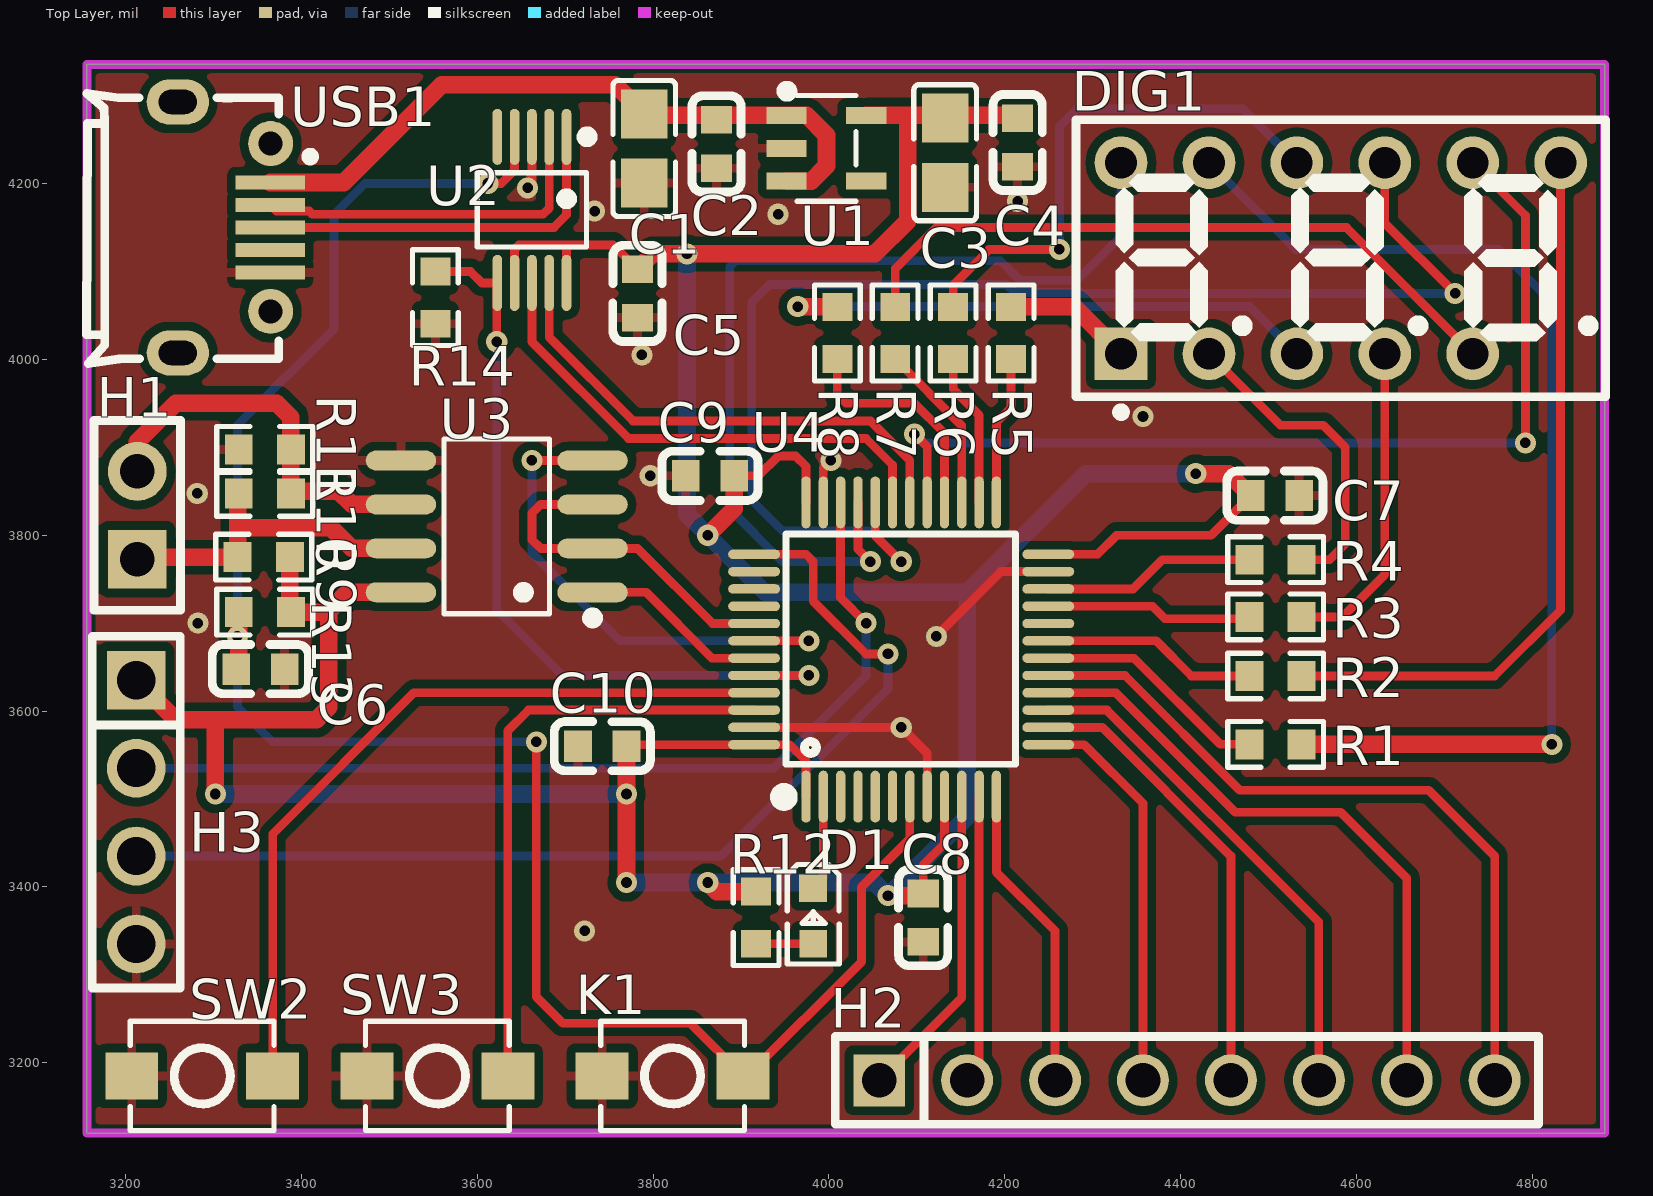
[diagram p0: Top Layer view]
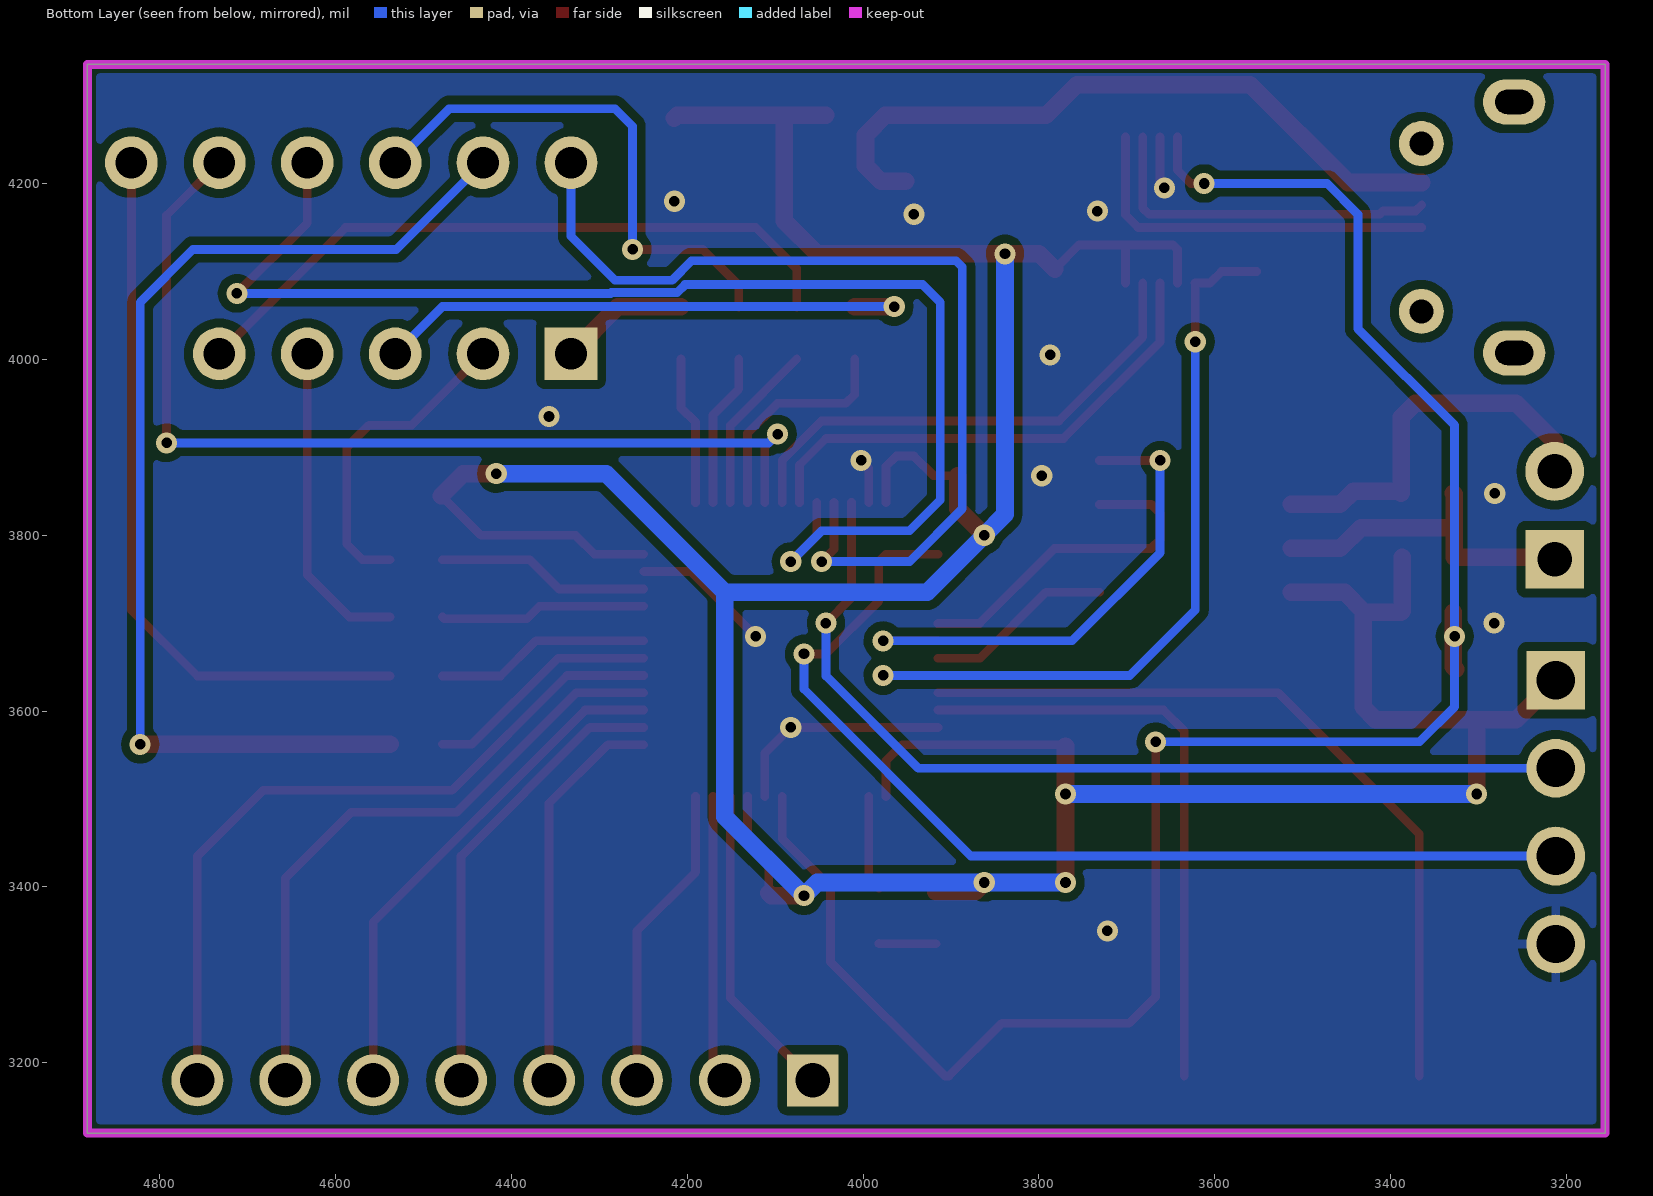
[diagram p1: Bottom Layer view, seen from below]
# Altium PCB MISC49919.pcbdoc
Units mil, origin at the board's own origin, x right, y up, seen from the top; angles counter-clockwise.
Board outline 1726.16 x 1215.5 mil, 2 copper layers (Top Layer, Bottom Layer), stack 62.206 mil thick; 37 components, 48 nets, 161 pads, 38 vias.

## Layer stack, top to bottom
Top Solder Mask Layer: solder mask 0.394, Dk 3.3
Top Layer: signal copper 1.379
Dielectric1: surface 59.449, FR4, Dk 4.5
Bottom Layer: signal copper 1.378
Bottom Solder Mask Layer: solder mask 0.394, Dk 3.3

## Board outline
3156.11,4335.5 3156.11,3120 4882.28,3120 4882.28,4335.5

## Design rules (kind name [scope] priority, off if disabled: settings)
BoardOutlineClearance copperThickness2oz_1 [All] p2 off: genericclearance=7.99 ignorepadtopadclearanceinfootprint=FALSE except(0: Arc-SplitContinuation Track-SplitContinuation SMDPad-SplitContinuation THPad-SplitContinuation Via-SplitContinuation Fill-SplitContinuation Region-SplitContinuation Poly-SplitContinuation Text-SplitContinuation Hole-SplitContinuation; 5.98: Arc-CutoutEdge SMDPad-CutoutEdge THPad-CutoutEdge Via-CutoutEdge Fill-CutoutEdge Region-CutoutEdge Text-CutoutEdge; 6.93: Hole-OutlineEdge Hole-CutoutEdge; 10: Poly-OutlineEdge Poly-CutoutEdge; 11.81: Arc-OutlineEdge Track-OutlineEdge SMDPad-OutlineEdge THPad-OutlineEdge Via-OutlineEdge Fill-OutlineEdge Region-OutlineEdge Text-OutlineEdge Track-CutoutEdge)
BoardOutlineClearance copperThickness1oz_1 [All] p4: genericclearance=4.02 ignorepadtopadclearanceinfootprint=FALSE except(0: Arc-SplitContinuation Track-SplitContinuation SMDPad-SplitContinuation THPad-SplitContinuation Via-SplitContinuation Fill-SplitContinuation Region-SplitContinuation Poly-SplitContinuation Text-SplitContinuation Hole-SplitContinuation; 6: SMDPad-CutoutEdge THPad-CutoutEdge Via-CutoutEdge Fill-CutoutEdge Region-CutoutEdge Text-CutoutEdge; 6.93: Hole-OutlineEdge Hole-CutoutEdge; 10: Poly-OutlineEdge Poly-CutoutEdge; 11.8: Arc-OutlineEdge Track-OutlineEdge SMDPad-OutlineEdge THPad-OutlineEdge Via-OutlineEdge Fill-OutlineEdge Region-OutlineEdge Text-OutlineEdge; 11.81: Arc-CutoutEdge Track-CutoutEdge)
Clearance copperThickness2oz [All] p1 off: gap=7.99 ignorepadtopadclearanceinfootprint=FALSE except(5.98: SMDPad-Track SMDPad-SMDPad THPad-Track SMDPad-THPad THPad-THPad Track-Via SMDPad-Via THPad-Via Via-Via Fill-Track Region-Track Fill-SMDPad Region-SMDPad Fill-THPad Region-THPad Fill-Via Region-Via Fill-Fill Fill-Region Region-Region Arc-Track Arc-SMDPad Arc-THPad Arc-Via Fill-Arc Region-Arc Arc-Arc Text-Track SMDPad-Text Text-THPad Text-Via Fill-Text Region-Text Arc-Text Text-Text; 6.93: Hole-Track Hole-SMDPad Hole-THPad Hole-Via Fill-Hole Region-Hole Hole-Arc Hole-Text; 10: Poly-Track Poly-SMDPad Poly-THPad Poly-Via Poly-Fill Poly-Region Poly-Poly Poly-Arc Poly-Text Poly-Hole)
Clearance copperThickness1oz [All] p3: gap=4.02 ignorepadtopadclearanceinfootprint=FALSE except(5.98: SMDPad-Track SMDPad-SMDPad THPad-Track SMDPad-THPad THPad-THPad Track-Via SMDPad-Via THPad-Via Via-Via Fill-Track Region-Track Fill-SMDPad Region-SMDPad Fill-THPad Region-THPad Fill-Via Region-Via Fill-Fill Fill-Region Region-Region; 6: Arc-Track Arc-SMDPad Arc-THPad Arc-Via Fill-Arc Region-Arc Arc-Arc Text-Track SMDPad-Text Text-THPad Text-Via Fill-Text Region-Text Arc-Text Text-Text; 6.93: Hole-Track Hole-SMDPad Hole-THPad Hole-Via Fill-Hole Region-Hole Hole-Arc Hole-Text; 10: Poly-Track Poly-SMDPad Poly-THPad Poly-Via Poly-Fill Poly-Region Poly-Poly Poly-Arc Poly-Text Poly-Hole)
DiffPairsRouting differentialPair [All] p1: maxlimit=6 minlimit=6 mostfreqgap=6 toplayer_minwidth=5 toplayer_prefwidth=10 toplayer_maxwidth=100 toplayer_mingap=6 toplayer_prefgap=6 toplayer_maxgap=6 bottomlayer_minwidth=5 bottomlayer_prefwidth=10 bottomlayer_maxwidth=100 bottomlayer_mingap=6 bottomlayer_prefgap=6 bottomlayer_maxgap=6 maxuncoupledlength=10
HoleToHoleClearance otherClearance [All] p1: gap=11.81 allowstackedmicrovias=TRUE
Length netLength [All] p1: minlimit=0 maxlimit=0
MatchedLengths netLengthTolerance [All] p1: tolerance=1000
PasteMaskExpansion pasteMaskExpansion [All] p1: expansion=0
PlaneConnect innerPlane [All] p1: planeconnectstyle=Relief reliefexpansion=20 reliefentries=4 reliefconductorwidth=10 reliefairgap=10
PolygonConnect copperRegion [(InNet('GND'))] p1: connectstyle=Relief reliefconductorwidth=10 reliefentries=4 polygonreliefangle="90 Angle" airgapwidth=10 via.connectstyle=Relief via.reliefconductorwidth=10 via.reliefentries=4 via.polygonreliefangle="90 Angle" via.airgapwidth=10
RoutingVias viaSize [All] p1: holewidth=12.01 width=24.02 viastyle="Through Hole" minholewidth=11.81 minwidth=19.68 maxholewidth=248.03 maxwidth=393.7
SolderMaskExpansion solderMaskExpansion [IsVia] p1: expansion=-1000 istentingtop=TRUE
SolderMaskExpansion solderMaskExpansion [All] p2: expansion=2 istentingtop=FALSE
Width copperThickness2oz_2 [All] p1 off: maxlimit=100 minlimit=8 preferedwidth=10
Width copperThickness1oz_2 [All] p2: maxlimit=100 minlimit=5 preferedwidth=10

## Components (designator, comment, footprint, x,y, rotation, side; value= is the part's Value field where it differs from the comment)
C1 "475" C0805 3790.02,4239.83 r90 top
C2 "104" C0603 3872.28,4245 r90 top
C3 "335" C0805 4132.28,4235 r90 top
C4 "104" C0603 4214.68,4246.64 r90 top
C5 "104" C0603 3782.28,4075 r90 top
C6 "104" C0603 3353.48,3647.6 r180 top
C7 "104" C0603 4507.28,3845 r180 top
C8 "104" C0603 4107.28,3365 r90 top
C9 "104" C0603 3864.84,3867.56 r0 top
C10 "104" C0603 3742.28,3560 r0 top
D1 "" LED_0603 3982.28,3365 r270 top
DIG1 "FJ2352AH" LED-SEG-TH_FJ2352AH 4582.28,4115 r0 top
H1 "" HDR-TH_2P-P2.54-V-F 3213.48,3822.6 r90 top
H2 "B-2100S08P-A110" HDR-TH_8P-P2.54-V-M 4407.28,3180 r0 top
H3 "PZ254V-11-04P" HDR-TH_4P-P2.54-V-M 3212.28,3485 r270 top
K1 "HX 3x4x2-2P-2.5N" SW-SMD_L4.0-W2.9-LS5.0 3822.28,3185 r0 top
R1 "1K" R0603 4508.12,3562.15 r180 top
R2 "1K" R0603 4508.12,3639.85 r180 top
R3 "1K" R0603 4508.12,3707.09 r180 top
R4 "1K" R0603 4508.12,3772.09 r180 top
R5 "1K" R0603 4207.28,4030 r270 top
R6 "1K" R0603 4141.38,4030 r270 top
R7 "1K" R0603 4075.49,4030 r270 top
R8 "1K" R0603 4009.6,4030 r270 top
R9 "10K" R0603 3357.28,3775 r180 top
R10 "120" R0603 3358.48,3847.6 r180 top
R11 "10K" R0603 3358.48,3897.6 r0 top
R12 "1K" R0603 3917.28,3365 r270 top
R13 "10K" R0603 3358.48,3712.6 r0 top
R14 "4.7K" R0603 3552.48,4070.16 r90 top
SW2 "HX 3x4x2-2P-2.5N" SW-SMD_L4.0-W2.9-LS5.0 3287.28,3185 r0 top
SW3 "HX 3x4x2-2P-2.5N" SW-SMD_L4.0-W2.9-LS5.0 3554.78,3185 r0 top
U1 "ME6211C33M5G-N" SOT-23-5_L3.0-W1.7-P0.95-LS2.8-BL 3997.28,4240 r270 top
U2 "CH340X" MSOP-10_L3.0-W3.0-P0.50-LS5.0-BL 3662.28,4170 r180 top
U3 "SP3485EEN(UMW)" SOP-8_L5.0-W4.0-P1.27-LS6.0-BL 3622.28,3810 r90 top
U4 "STM32F103C6T6ATR" LQFP-48_L7.0-W7.0-P0.50-LS9.0-BL 4082.28,3670 r0 top
USB1 "MicroXNJ" MICRO-USB-SMD_MICROXNJ_1 3312.28,4150 r270 top

## Footprints (in the part's own frame and the unit in brackets; to place one, negate y for a bottom-side part, rotate by r counter-clockwise, add the part's x,y. Pads: shape width x height; smd on the part's side, far side on the other; paste and mask are expansions set on the pad)
C0603 [mm]
  rect 0.8x0.9 smd: 1(-0.7,0) 2(0.7,0)
  silkscreen extent -1.39,-0.71 1.39,0.71
C0805 [mm]
  rect 1.41x1.35 smd paste-100 mask+0.051: 1(-1,0) 2(1,0)
  silkscreen extent -1.96,-0.9 1.96,0.9
HDR-TH_2P-P2.54-V-F [mm]
  rect 1.7x1.7 hole 1: 1(-1.27,0)
  round 1.7 hole 1: 2(1.27,0)
  silkscreen extent -2.74,-1.25 2.74,1.25
HDR-TH_4P-P2.54-V-M [mm]
  rect 1.7x1.7 hole 1.1: 1(-3.81,0)
  round 1.7 hole 1.1: 2(-1.27,0) 3(1.27,0) 4(3.81,0)
  silkscreen extent -5.08,-1.27 5.08,1.27
HDR-TH_8P-P2.54-V-M [mm]
  rect 1.5x1.5 hole 1: 1(-8.89,0)
  round 1.5 hole 1: 2(-6.35,0) 3(-3.81,0) 4(-1.27,0) 5(1.27,0) 6(3.81,0) 7(6.35,0) 8(8.89,0)
  silkscreen extent -10.16,-1.27 10.16,1.27
LED-SEG-TH_FJ2352AH [mil]
  rect 60x60 hole 36: 1(-250,-108.66)
  round 60 hole 36: 2(-150,-108.66) 3(-50,-108.66) 4(50,-108.66) 5(150,-108.66) 7(250,108.66) 8(150,108.66) 9(50,108.66) 10(-50,108.66) 11(-150,108.66) 12(-250,108.66)
  silkscreen extent -301,-180 301,157
LED_0603 [mil]
  rect 31.5x31.5 smd paste+0 mask+2: 1(-33.5,-0.4) 2(29.5,-0.2)
  silkscreen extent -61,-30 53,30
LQFP-48_L7.0-W7.0-P0.50-LS9.0-BL [mm]
  oval 0.27x1.5 smd paste+0 mask+0.05: 1(-2.75,-4.25) 2(-2.25,-4.25) 3(-1.75,-4.25) 4(-1.25,-4.25) 5(-0.75,-4.25) 6(-0.25,-4.25) 7(0.25,-4.25) 8(0.75,-4.25) 9(1.25,-4.25) 10(1.75,-4.25) 11(2.25,-4.25) 12(2.75,-4.25) 25(2.75,4.25) 26(2.25,4.25) 27(1.75,4.25) 28(1.25,4.25) 29(0.75,4.25) 30(0.25,4.25) 31(-0.25,4.25) 32(-0.75,4.25) 33(-1.25,4.25) 34(-1.75,4.25) 35(-2.25,4.25) 36(-2.75,4.25)
  oval 1.5x0.27 smd paste+0 mask+0.05: 13(4.25,-2.75) 14(4.25,-2.25) 15(4.25,-1.75) 16(4.25,-1.25) 17(4.25,-0.75) 18(4.25,-0.25) 19(4.25,0.25) 20(4.25,0.75) 21(4.25,1.25) 22(4.25,1.75) 23(4.25,2.25) 24(4.25,2.75) 37(-4.25,2.75) 38(-4.25,2.25) 39(-4.25,1.75) 40(-4.25,1.25) 41(-4.25,0.75) 42(-4.25,0.25) 43(-4.25,-0.25) 44(-4.25,-0.75) 45(-4.25,-1.25) 46(-4.25,-1.75) 47(-4.25,-2.25) 48(-4.25,-2.75)
  silkscreen extent -3.59,-4.46 3.3,3.34
MICRO-USB-SMD_MICROXNJ_1 [mm]
  rect 0.4x2 smd paste-100 mask+0.051: 1(-1.3,1.332) 2(-0.65,1.332) 3(0,1.332) 4(0.65,1.332) 5(1.3,1.332)
  round 1.3 hole 0.7 paste+0 mask+0.051: 6(2.425,1.34)
  oval 1.3x1.8 hole 0.7 slot 1.1 at 90 deg: 7(3.625,-1.34) 8(-3.625,-1.34)
  round 1.3 hole 0.7: 9(-2.425,1.34)
  Inner2 circle w0.1: c-3.886,-7.882 r0.05
  silkscreen extent -3.87,-3.98 3.93,2.61
MSOP-10_L3.0-W3.0-P0.50-LS5.0-BL [mm]
  oval 0.28x1.62 smd: 1(-1,-2.11) 2(-0.5,-2.11) 3(0,-2.11) 4(0.5,-2.11) 5(1,-2.11) 6(1,2.11) 7(0.5,2.11) 8(0,2.11) 9(-0.5,2.11) 10(-1,2.11)
  silkscreen extent -1.74,-2.26 1.58,1.07
R0603 [mil]
  rect 31.75x34.02 smd paste-3937.01 mask+2: 1(-29.66,0) 2(29.66,0)
  silkscreen extent -55,-26 55,26
SOP-8_L5.0-W4.0-P1.27-LS6.0-BL [mil]
  oval 22.6x80.14 smd: 1(-75,-108.97) 2(-25,-108.97) 3(25,-108.97) 4(75,-108.97) 5(75,108.97) 6(25,108.97) 7(-25,108.97) 8(-75,108.97)
  silkscreen extent -110,-115 99,60
SOT-23-5_L3.0-W1.7-P0.95-LS2.8-BL [mm]
  rect 0.49x1.157 smd: 1(-0.95,-1.154) 2(0,-1.154) 3(0.95,-1.154)
  rect 0.49x1.175 smd: 4(0.95,1.154) 5(-0.95,1.154)
  silkscreen extent -1.8,-1.29 1.53,0.85
SW-SMD_L4.0-W2.9-LS5.0 [mm]
  rect 1.53x1.36 smd: 1(-2.035,0) 2(2.035,0)
  silkscreen extent -2.08,-1.58 2.08,1.58

## Via types
v1: diameter 24.02, hole 12, Top Layer to Bottom Layer, 38 vias

## Nets (pads, with @x,y where several pads share a name; then routed paths per layer and width w, separated by ;. In a path a pad name is that pad's centre, name@x,y a point inside that pad or via, vN(x,y) a via of type N, cw(c..) or ccw(c..) an arc to the next point about the centre after c; other vN are vias at no path point)
485_RX: U3.1 U4.43 | length 214.7
  Top Layer w10: U3.1 3792.28,3735 3867.12,3660.16 U4.43
485_TX: U3.4 U4.42 | length 592.8
  Top Layer w10: v1(3662.28,3885) U3.4 ; U4.42 v1(3977.28,3679.84)
  Bottom Layer w10: v1(3662.28,3885) 3662.28,3780 3762.44,3679.84 v1(3977.28,3679.84)
$1N39: H1.1 R9.2 R10.2 U3.7 | length 383.7
  Top Layer w20: H1.1 3215.88,3775 R9.2 3327.62,3808.55 ; R10.2 3327.62,3846.4 3327.62,3808.55 ; U3.7 3457.28,3785 3433.73,3808.55 3327.62,3808.55
$1N40: H1.2 R10.1 R11.2 U3.6 | length 451.9
  Top Layer w20: H1.2 3213.48,3906.2 3257.28,3950 3372.28,3950 3388.14,3934.14 R11.2 R10.1 3390.54,3850 3442.28,3850 3457.28,3835 U3.6
$1N56: D1.1 U4.2 | length 109.1
  Top Layer w10: D1.1 3993.7,3410.32 U4.2
$1N57: D1.2 R12.2 | length 64.9
  Top Layer w10: R12.2 3981.92,3335.34 D1.2
+5V: C1.2 C2.2 U1.1 U1.3 USB1.1 | length 789.9
  Top Layer w20: USB1.1 3448.46,4201.18 3559.57,4312.29 3756.92,4312.29 C1.2 3791.81,4277.4 U1.1 3974.88,4277.4 3997.28,4255 3997.28,4220 3979.88,4202.6 U1.3
A: DIG1.11 R1.1 | length 1243.1
  Top Layer w20: R1.1 v1(4822.28,3562.15)
  Bottom Layer w10: DIG1.11 4530.94,4125 4762.28,4125 4822.28,4065 v1(4822.28,3562.15)
B: DIG1.7 R2.1 | length 834.3
  Top Layer w10: R2.1 4757.12,3639.85 4832.28,3715 DIG1.7
BOOT0: R14.2 U2.6 U4.44 | length 896.1
  Top Layer w10: R14.2 3592.45,4099.82 3605.35,4086.93 U2.6 3622.28,4086.3 v1(3622.28,4020) ; U4.44 v1(3977.28,3640.47)
  Bottom Layer w10: v1(3622.28,4020) 3622.28,3715 3696.81,3640.47 v1(3977.28,3640.47)
BOOT1: U4.20
C: DIG1.4 R3.1 | length 365.7
  Top Layer w10: R3.1 4584.37,3707.09 4632.28,3755 DIG1.4
D: DIG1.2 R4.1 | length 366
  Top Layer w10: DIG1.2 4513.62,3925 4562.28,3925 4587.28,3900 4587.28,3790 4569.37,3772.09 R4.1
D+: U2.1 USB1.3 | length 431.6
  Top Layer w10: USB1.3 3687.28,4150 3701.65,4164.37 U2.1
D-: U2.2 USB1.2 | length 405.6
  Top Layer w10: USB1.2 3371.46,4168.86 3408.65,4168.86 3412.51,4165 3674.95,4165 3681.96,4172.01 U2.2
DIG1: DIG1.12 U4.33 | length 1094.5
  Top Layer w10: U4.33 4033.07,3784.21 v1(4047.28,3770)
  Bottom Layer w10: v1(4047.28,3770) 3947.28,3770 3887.28,3830 3887.28,4105 3894.35,4112.07 4195.21,4112.07 4217.28,4090 4282.28,4090 4332.28,4140 DIG1.12
DIG2: DIG1.9 U4.32 | length 1497.8
  Top Layer w10: U4.32 4052.75,3799.53 v1(4082.28,3770) ; DIG1.9 4632.28,4155 v1(4712.28,4075)
  Bottom Layer w10: v1(4082.28,3770) 4047.28,3805 3947.28,3805 3912.28,3840 3912.28,4065 3932.28,4085 4202.46,4085 4211.47,4075.98 4286.29,4075.98 4287.28,4075 v1(4712.28,4075)
DIG3: DIG1.8 U4.29 | length 1126.4
  Top Layer w10: v1(4097.28,3915) 4111.81,3900.47 U4.29 ; DIG1.8 4792.28,4163.66 v1(4792.28,3905)
  Bottom Layer w10: v1(4097.28,3915) 4107.28,3905 v1(4792.28,3905)
DP: DIG1.3 R8.1 | length 635
  Top Layer w20: v1(3964.6,4060) 4009.26,4060 R8.1
  Bottom Layer w10: v1(3964.6,4060) 4478.62,4060 DIG1.3
E: DIG1.1 R5.1 | length 147.1
  Top Layer w20: R5.1 4278.96,4059.66 DIG1.1
F: DIG1.10 R6.1 | length 606
  Top Layer w10: R6.1 4141.38,4084.11 4182.28,4125 v1(4262.28,4125)
  Bottom Layer w10: v1(4262.28,4125) 4262.28,4265 4282.28,4285 4470.94,4285 DIG1.10
G: DIG1.5 R7.1 | length 779.2
  Top Layer w10: R7.1 4075.49,4103.21 4122.28,4150 4588.62,4150 DIG1.5
GND: C1.1 C2.1 C3.1 C4.1 C5.1 C6.1 C7.1 C8.1 C9.1 C10.1 H3.4 K1.1 R11.1 R14.1 SW2.1 SW3.1 U1.2 U2.3 U3.5 U4.8 U4.23 U4.35 U4.47 USB1.5 | length 527.5
  Top Layer w10: v1(3657.28,4195) 3662.28,4200 U2.3 ; U4.47 v1(4082.28,3581.42) 4111.81,3551.89 U4.8 ; U4.35 3993.7,3876.42 v1(4002.28,3885) ; v1(4122.28,3685) 4195.86,3758.58 U4.23
  other v1: 3722.28,3350 3282.28,3700 3281.62,3847.6 3796.82,3867.55 4357.28,3935 3787.28,4005 3942.28,4165 3733.61,4168.52 4214.68,4179.83
KEY0: SW2.2 U4.45 | length 889.2
  Top Layer w10: SW2.2 3367.4,3460.12 3528.07,3620.79 U4.45
KEY1: SW3.2 U4.46 | length 682.4
  Top Layer w10: SW3.2 3634.9,3577.62 3658.38,3601.1 U4.46
PA0: H2.1 U4.10 | length 361.6
  Top Layer w10: H2.1 4151.18,3273.9 U4.10
PA1: H2.2 U4.11 | length 328.3
  Top Layer w10: H2.2 4170.86,3193.58 U4.11
PA2: H2.3 U4.12 | length 350.3
  Top Layer w10: U4.12 4190.55,3416.73 4257.28,3350 H2.3
PA3: H2.4 U4.13 | length 450.3
  Top Layer w10: U4.13 4290.55,3561.73 4357.28,3495 H2.4
PA4: H2.5 U4.14 | length 523.3
  Top Layer w10: U4.14 4310.86,3581.42 4457.28,3435 H2.5
PA5: H2.6 U4.15 | length 587.5
  Top Layer w10: U4.15 4316.18,3601.1 4557.28,3360 H2.6
PA6: H2.7 U4.16 | length 725
  Top Layer w10: U4.16 4326.49,3620.79 4462.28,3485 4582.28,3485 4657.28,3410 H2.7
PA7: H2.8 U4.17 | length 847.8
  Top Layer w10: U4.17 4336.81,3640.47 4467.28,3510 4682.28,3510 4757.28,3435 H2.8
PB0: R1.2 U4.18 | length 269.5
  Top Layer w10: U4.18 4347.12,3660.16 4445.13,3562.15 R1.2
PB1: R2.2 U4.19 | length 245.4
  Top Layer w10: U4.19 4372.44,3679.84 4412.43,3639.85 R2.2
PB10: R3.2 U4.21 | length 235.6
  Top Layer w10: U4.21 4368.07,3719.21 4382.28,3705 4476.37,3705 R3.2
PB11: R4.2 U4.22 | length 242.6
  Top Layer w10: U4.22 4346.18,3738.9 4379.37,3772.09 R4.2
PB12: R5.2 U4.25 | length 169.9
  Top Layer w10: U4.25 4190.55,3928.27 4207.28,3945 R5.2
PB13: R6.2 U4.26 | length 175.2
  Top Layer w10: R6.2 4141.38,3965.89 4170.86,3936.42 U4.26
PB14: R7.2 U4.27 | length 194.4
  Top Layer w10: R7.2 4151.18,3924.65 U4.27
PB15: R8.2 U4.28 | length 259
  Top Layer w10: R8.2 4009.6,3960 4019.6,3950 4097.28,3950 4131.49,3915.79 U4.28
RESET: C6.2 K1.2 R13.1 U2.4 U4.7 | length 2253.8
  Top Layer w10: v1(3612.28,4200) 3627.28,4200 3642.59,4215.31 U2.4 ; v1(3667.28,3565) 3667.28,3275 3697.28,3245 3842.4,3245 K1.2 3907.28,3185 4037.28,3315 4037.28,3400 4092.12,3454.84 U4.7
  Top Layer w20: C6.2 3328.82,3650.5 R13.1
  Bottom Layer w10: v1(3612.28,4200) 3472.28,4200 3437.28,4165 3437.28,4035 3327.28,3925 v1(3327.28,3685) 3327.28,3605 3367.28,3565 v1(3667.28,3565)
SWCLK: H3.3 U4.37 | length 1199.3
  Top Layer w10: U4.37 3974.01,3778.27 3982.28,3770 3982.28,3725 4042.28,3665 v1(4067.28,3665)
  Bottom Layer w10: H3.3 3877.28,3435 4067.28,3625 v1(4067.28,3665)
SWDIO: H3.2 U4.34 | length 1082.8
  Top Layer w10: U4.34 4013.38,3728.9 v1(4042.28,3700)
  Bottom Layer w10: H3.2 3937.28,3535 4042.28,3640 v1(4042.28,3700)
TRC: U3.2 U3.3 U4.41 | length 395.3
  Top Layer w10: U3.3 3672.28,3835 3662.28,3825 3662.28,3795 3672.28,3785 U3.2 3782.28,3785 3867.75,3699.53 U4.41
USART1_RX: U2.8 U4.31 | length 577.7
  Top Layer w10: U2.8 3662.28,4020 3772.28,3910 4042.28,3910 4072.44,3879.84 U4.31
USART1_TX: U2.9 U4.30 | length 577.7
  Top Layer w10: U2.9 3681.96,4025.32 3777.28,3930 4047.28,3930 4092.12,3885.16 U4.30
VCC: C3.2 C4.2 C5.2 C7.2 C8.2 C9.2 C10.2 H3.1 R9.1 R12.1 R13.2 U1.5 U2.7 U2.10 U3.8 U4.1 U4.9 U4.24 U4.36 U4.48 | length 4791.3
  Top Layer w10: U2.7 3642.59,4125.31 3647.28,4130 3700.64,4130 ; U2.10 3701.65,4129 3700.64,4130 ; C10.2 3771.57,3561.73 U4.48 3955.55,3561.73 3974.01,3543.27 U4.1 ; C5.2 3754.84,4130 3700.64,4130 ; C9.2 3919.84,3867.56 3942.28,3890 3962.28,3890 3974.01,3878.27 U4.36 ; C8.2 4107.28,3425 4131.49,3449.21 U4.9 ; U4.24 4305.55,3778.27 4327.28,3800 4434.72,3800 C7.2
  Top Layer w20: H3.1 3257.28,3590 3298.57,3590 ; v1(3302.28,3505.64) 3302.28,3586.29 3298.57,3590 ; R9.1 3386.94,3713.8 R13.2 3429.88,3712.6 ; U3.8 3452.28,3735 3429.88,3712.6 ; v1(3769.84,3405) v1(3769.84,3505.64) C10.2 ; C5.2 3799.72,4120 v1(3838.63,4120) 4052.28,4120 4089.68,4157.4 4089.68,4277.4 ; v1(3862.28,3405) 3872.62,3394.66 R12.1 ; v1(3862.28,3800) 3892.4,3830.12 C9.2 ; U1.5 4089.68,4277.4 ; v1(4067.28,3390) 4104.72,3390 C8.2 ; C4.2 4211.48,4277.4 4089.68,4277.4 ; v1(4417.28,3870) 4454.72,3870 C7.2 ; 3298.57,3590 3417.28,3590 3431.42,3604.14 3431.42,3711.05 3429.88,3712.6
  Bottom Layer w20: v1(3302.28,3505.64) v1(3769.84,3505.64) ; v1(3769.84,3405) v1(3862.28,3405) 4052.28,3405 v1(4067.28,3390) 4157.28,3480 4157.28,3735 ; v1(3838.63,4120) 3838.63,3823.65 v1(3862.28,3800) 3927.28,3735 4157.28,3735 ; v1(4417.28,3870) 4292.28,3870 4157.28,3735
pads on no net: U1.4 U2.5 U4.3 U4.4 U4.5 U4.6 U4.38 U4.39 U4.40 USB1.4 USB1.6 USB1.7 USB1.8 USB1.9

## Polygon pours and split planes (outlines as drawn)
GND on Bottom Layer (solid, remove dead copper, pour order 2): 3017.28,4425 3017.28,3000 5027.28,3000 5027.28,4425
GND on Top Layer (solid, remove dead copper, pour order 0): 3057.28,4410 3057.28,3015 5002.28,3015 5002.28,4410

## Keep-outs
Board Outline Layer:
  the board outline again, w10